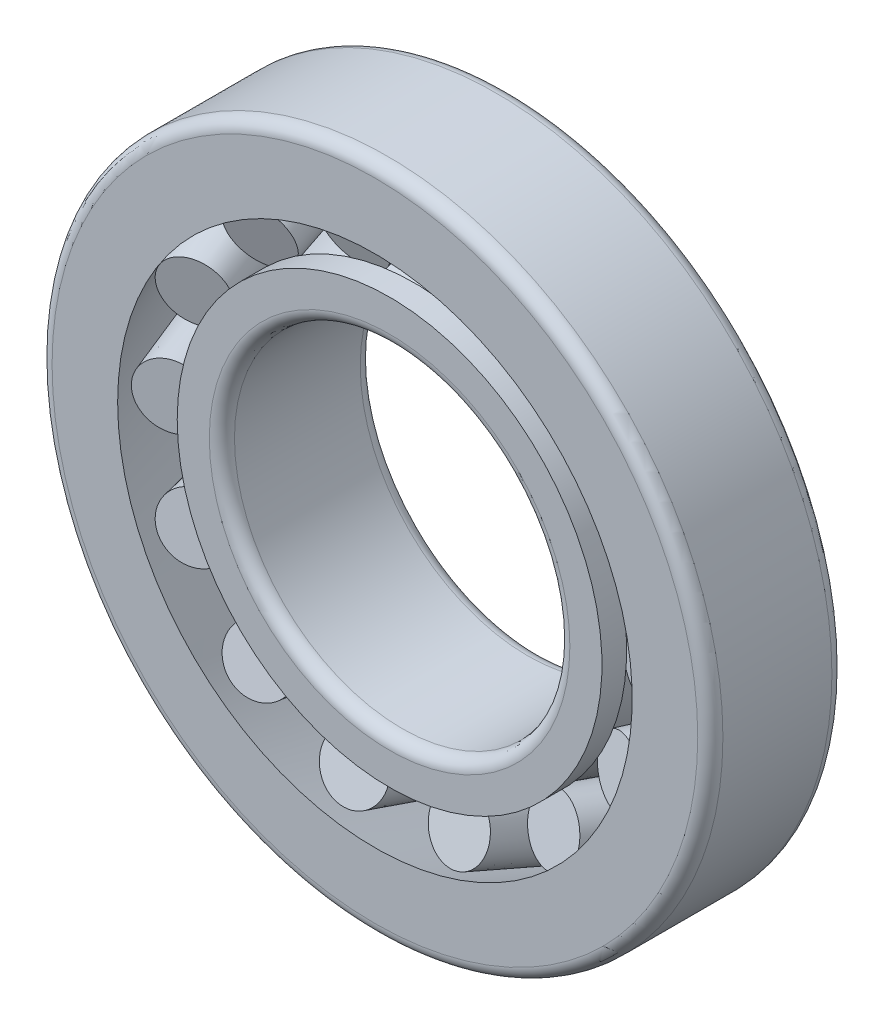
from build123d import *

# Parameters (mm, degrees)
PATTERN_CIRCULAR_1_COUNT = 14


with BuildPart() as part:
    # 草图1 → 旋转1 (revolve)
    with BuildSketch(Plane.XZ, mode=Mode.PRIVATE) as revolve_1_sk:
        with BuildLine():
            Line((28.735815031, 0), (21.5, 0))
            ThreePointArc((21.5, 0), (20.439339828, 0.439339828), (20, 1.5))
            Line((20, 1.5), (20, 16.5))
            ThreePointArc((20, 16.5), (20.439339828, 17.560660172), (21.5, 18))
            Line((21.5, 18), (25.326735538, 18))
            Line((25.326735538, 18), (25.326735538, 15.057777647))
            Line((25.326735538, 15.057777647), (24.363707186, 14.726736651))
            Line((24.363707186, 14.726736651), (27.772786678, 3.20941449))
            Line((27.772786678, 3.20941449), (28.735815031, 3.540455486))
            Line((28.735815031, 3.540455486), (28.735815031, 0))
        make_face()
    revolve(revolve_1_sk.sketch.rotate(Axis((0, 0, 0), (0, 0, 1)), 180), axis=Axis((0, 0, 0), (0, 0, 1)))


with BuildPart() as body_2:
    # 草图2 → 旋转2 (revolve)
    with BuildSketch(Plane(origin=(30, 0, 10.3125), x_dir=(0, -1, 0), z_dir=(-0.9456865993048664, 0, -0.3250797685110486)), mode=Mode.PRIVATE) as revolve_2_sk:
        Polygon((0, -5.94), (4.302664453, -5.94), (3.777335547, 5.94), (0, 5.94), align=None)
    revolve(revolve_2_sk.sketch.rotate(Axis((30, 0, 10.3125), (-0.32507976851104853, 0, 0.9456865993048665)), 270), axis=Axis((30, 0, 10.3125), (-0.32507976851104853, 0, 0.9456865993048665)))


with BuildPart() as body_3:
    # 草图3 → 旋转3 (revolve)
    with BuildSketch(Plane.XZ, mode=Mode.PRIVATE) as revolve_3_sk:
        with BuildLine():
            Line((36.968820734, 3.75), (38.500000001, 3.75))
            ThreePointArc((38.500000001, 3.75), (39.560660173, 4.189339828), (40.000000001, 5.25))
            Line((40.000000001, 5.25), (40.000000001, 18.25))
            ThreePointArc((40.000000001, 18.25), (39.560660173, 19.310660172), (38.500000001, 19.75))
            Line((38.500000001, 19.75), (30.681641467, 19.75))
            Line((30.681641467, 19.75), (36.968820734, 3.75))
        make_face()
    revolve(revolve_3_sk.sketch.rotate(Axis((0, 0, 0), (0, 0, 1)), 180), axis=Axis((0, 0, 0), (0, 0, 1)))


with BuildPart() as pattern_circular_1_1:
    # 阵列(圆周)1: pattern copy
    add(body_2.part.rotate(Axis((0, 0, 0), (0, 0, 1)), 1 * 360 / PATTERN_CIRCULAR_1_COUNT))


with BuildPart() as pattern_circular_1_2:
    # 阵列(圆周)1: pattern copy
    add(body_2.part.rotate(Axis((0, 0, 0), (0, 0, 1)), 2 * 360 / PATTERN_CIRCULAR_1_COUNT))


with BuildPart() as pattern_circular_1_3:
    # 阵列(圆周)1: pattern copy
    add(body_2.part.rotate(Axis((0, 0, 0), (0, 0, 1)), 3 * 360 / PATTERN_CIRCULAR_1_COUNT))


with BuildPart() as pattern_circular_1_4:
    # 阵列(圆周)1: pattern copy
    add(body_2.part.rotate(Axis((0, 0, 0), (0, 0, 1)), 4 * 360 / PATTERN_CIRCULAR_1_COUNT))


with BuildPart() as pattern_circular_1_5:
    # 阵列(圆周)1: pattern copy
    add(body_2.part.rotate(Axis((0, 0, 0), (0, 0, 1)), 5 * 360 / PATTERN_CIRCULAR_1_COUNT))


with BuildPart() as pattern_circular_1_6:
    # 阵列(圆周)1: pattern copy
    add(body_2.part.rotate(Axis((0, 0, 0), (0, 0, 1)), 6 * 360 / PATTERN_CIRCULAR_1_COUNT))


with BuildPart() as pattern_circular_1_7:
    # 阵列(圆周)1: pattern copy
    add(body_2.part.rotate(Axis((0, 0, 0), (0, 0, 1)), 7 * 360 / PATTERN_CIRCULAR_1_COUNT))


with BuildPart() as pattern_circular_1_8:
    # 阵列(圆周)1: pattern copy
    add(body_2.part.rotate(Axis((0, 0, 0), (0, 0, 1)), 8 * 360 / PATTERN_CIRCULAR_1_COUNT))


with BuildPart() as pattern_circular_1_9:
    # 阵列(圆周)1: pattern copy
    add(body_2.part.rotate(Axis((0, 0, 0), (0, 0, 1)), 9 * 360 / PATTERN_CIRCULAR_1_COUNT))


with BuildPart() as pattern_circular_1_10:
    # 阵列(圆周)1: pattern copy
    add(body_2.part.rotate(Axis((0, 0, 0), (0, 0, 1)), 10 * 360 / PATTERN_CIRCULAR_1_COUNT))


with BuildPart() as pattern_circular_1_11:
    # 阵列(圆周)1: pattern copy
    add(body_2.part.rotate(Axis((0, 0, 0), (0, 0, 1)), 11 * 360 / PATTERN_CIRCULAR_1_COUNT))


with BuildPart() as pattern_circular_1_12:
    # 阵列(圆周)1: pattern copy
    add(body_2.part.rotate(Axis((0, 0, 0), (0, 0, 1)), 12 * 360 / PATTERN_CIRCULAR_1_COUNT))


with BuildPart() as pattern_circular_1_13:
    # 阵列(圆周)1: pattern copy
    add(body_2.part.rotate(Axis((0, 0, 0), (0, 0, 1)), 13 * 360 / PATTERN_CIRCULAR_1_COUNT))


solid = Compound([part.part, body_2.part, body_3.part, pattern_circular_1_1.part, pattern_circular_1_2.part, pattern_circular_1_3.part, pattern_circular_1_4.part, pattern_circular_1_5.part, pattern_circular_1_6.part, pattern_circular_1_7.part, pattern_circular_1_8.part, pattern_circular_1_9.part, pattern_circular_1_10.part, pattern_circular_1_11.part, pattern_circular_1_12.part, pattern_circular_1_13.part])
